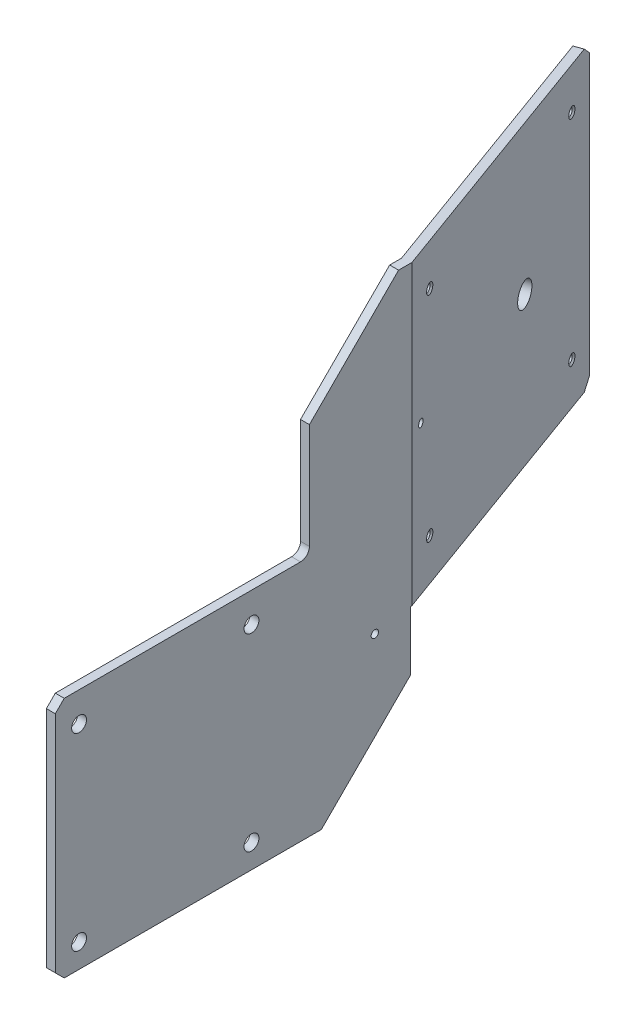
from build123d import *

# Parameters (mm, degrees)
BOSS_EXTRUDE1_DEPTH   = 100
SKETCH3_R             = 1
CUT_EXTRUDE2_DEPTH    = 10
LPATTERN1_COUNT       = 2
LPATTERN1_PITCH       = 80
M3_TAPPED_HOLE1_D     = 2.5
M3_TAPPED_HOLE1_DEPTH = 7.5
M3_TAPPED_HOLE1_TIP   = 0.751075774
CHAMFER2_SIZE         = 0.5
SKETCH6_W             = 85.5
SKETCH6_H             = 68.5
CUT_EXTRUDE4_DEPTH    = 10
CHAMFER3_SIZE         = 30
FILLET1_R             = 3
SKETCH7_R             = 4
CUT_EXTRUDE5_DEPTH    = 10
SKETCH9_W             = 119.5
SKETCH9_H             = 50
BOSS_EXTRUDE2_DEPTH   = 3
SKETCH5_R             = 2.5
CUT_EXTRUDE3_DEPTH    = 10
CHAMFER4_SIZE         = 3
CHAMFER5_SIZE         = 30
M3_TAPPED_HOLE2_D     = 2.5
M3_TAPPED_HOLE2_DEPTH = 7.5
M3_TAPPED_HOLE2_TIP   = 0.751075774
M3_TAPPED_HOLE3_D     = 2.5
M3_TAPPED_HOLE3_DEPTH = 7.5
M3_TAPPED_HOLE3_TIP   = 0.751075774


with BuildPart() as part:
    # Sketch1 → Boss-Extrude1 (new body)
    with BuildSketch(Plane(origin=(0, 0, 0), x_dir=(1, 0, 0), z_dir=(0, 1, 0))):
        Polygon((0, 120), (-34.202014333, 213.969262079), (-37.021092195, 212.943201649), (-3, 119.471019058), (-3, 0), (0, 0), align=None)
    extrude(amount=BOSS_EXTRUDE1_DEPTH)

    # Sketch3 → Cut-Extrude2 (cut)
    with BuildSketch(Plane(origin=(35.748178719, 0, -13.011272983), x_dir=(0.3420201433256699, 0, 0.939692620785908), z_dir=(-0.9396926207859081, 0, 0.3420201433256699))):
        with Locations((-202.763114494, 86)):
            Circle(SKETCH3_R)
        with Locations((-202.763114494, 14)):
            Circle(SKETCH3_R)
    cut_extrude2 = extrude(amount=-CUT_EXTRUDE2_DEPTH, mode=Mode.SUBTRACT)

    # LPattern1: Cut-Extrude2 ×2
    with Locations(*[Vector(0.3420201433256699, 0, 0.939692620785908) * (i * LPATTERN1_PITCH) for i in range(1, LPATTERN1_COUNT)]):
        add(cut_extrude2, mode=Mode.SUBTRACT)

    # M3 Tapped Hole1
    with Locations(Plane(origin=(-30.781812899, 86, -204.572335871), x_dir=(0.342020143326, 0, 0.939692620786), z_dir=(0.939692620786, 0, -0.342020143326))):
        with Locations((0, 0), (0, 72), (80, 72), (80, 0)):
            Hole(M3_TAPPED_HOLE1_D / 2, depth=M3_TAPPED_HOLE1_DEPTH)
            with Locations((0, 0, -(M3_TAPPED_HOLE1_DEPTH + M3_TAPPED_HOLE1_TIP / 2))):  # 118° drill point
                Cone(0, M3_TAPPED_HOLE1_D / 2, M3_TAPPED_HOLE1_TIP, mode=Mode.SUBTRACT)

    # Chamfer2
    chamfer2_edges = [part.edges().sort_by_distance(p)[0] for p in [
        (-2.992676254, 86, -128.222310432),
        (-2.992676254, 14, -128.222310432),
        (-30.35428772, 14, -203.397720095),
        (-30.35428772, 86, -203.397720095),
    ]]
    chamfer(chamfer2_edges, length=CHAMFER2_SIZE)

    # Sketch6 → Cut-Extrude4 (cut)
    with BuildSketch(Plane.ZY.offset(3)):
        with Locations((-42.75, 65.75)):
            Rectangle(SKETCH6_W, SKETCH6_H)
    extrude(amount=-CUT_EXTRUDE4_DEPTH, mode=Mode.SUBTRACT)

    # Chamfer3
    chamfer3_edges = [part.edges().sort_by_distance(p)[0] for p in [
        (-1.5, 100, -85.5),
    ]]
    chamfer(chamfer3_edges, length=CHAMFER3_SIZE)

    # Fillet1
    fillet1_edges = [part.edges().sort_by_distance(p)[0] for p in [
        (-1.5, 31.5, -85.5),
    ]]
    fillet(fillet1_edges, radius=FILLET1_R)

    # Sketch7 → Cut-Extrude5 (cut)
    with BuildSketch(Plane(origin=(35.748178719, 0, -13.011272983), x_dir=(0.3420201433256699, 0, 0.939692620785908), z_dir=(-0.9396926207859081, 0, 0.3420201433256699))):
        with Locations((-176.263114494, 50)):
            Circle(SKETCH7_R)
    extrude(amount=-CUT_EXTRUDE5_DEPTH, mode=Mode.SUBTRACT)

    # Sketch9 → Boss-Extrude2 (add)
    with BuildSketch(Plane.ZY.offset(3)):
        with Locations((-59.75, -25)):
            Rectangle(SKETCH9_W, SKETCH9_H)
    extrude(amount=-BOSS_EXTRUDE2_DEPTH)

    # Sketch5 → Cut-Extrude3 (cut)
    with BuildSketch(Plane.ZY.offset(3)):
        with Locations((-8, 21.5)):
            Circle(SKETCH5_R)
        with Locations((-8, -42)):
            Circle(SKETCH5_R)
        with Locations((-66, 21.5)):
            Circle(SKETCH5_R)
        with Locations((-66, -42)):
            Circle(SKETCH5_R)
    extrude(amount=-CUT_EXTRUDE3_DEPTH, mode=Mode.SUBTRACT)

    # Chamfer4
    chamfer4_edges = [part.edges().sort_by_distance(p)[0] for p in [
        (-1.5, 31.5, 0),
        (-35.611553264, 100, -213.456231864),
        (-35.611553264, 0, -213.456231864),
        (-1.5, -50, 0),
    ]]
    chamfer(chamfer4_edges, length=CHAMFER4_SIZE)

    # Chamfer5
    chamfer5_edges = [part.edges().sort_by_distance(p)[0] for p in [
        (-1.5, -50, -119.5),
    ]]
    chamfer(chamfer5_edges, length=CHAMFER5_SIZE)

    # M3 Tapped Hole2
    with Locations(Plane(origin=(35.748178719, 0, -13.011272983), x_dir=(0.3420201433256699, 0, 0.939692620785908), z_dir=(-0.9396926207859081, 0, 0.3420201433256699))):
        with Locations((-117.763114494, 50)):
            Hole(M3_TAPPED_HOLE2_D / 2, depth=M3_TAPPED_HOLE2_DEPTH)
            with Locations((0, 0, -(M3_TAPPED_HOLE2_DEPTH + M3_TAPPED_HOLE2_TIP / 2))):  # 118° drill point
                Cone(0, M3_TAPPED_HOLE2_D / 2, M3_TAPPED_HOLE2_TIP, mode=Mode.SUBTRACT)

    # M3 Tapped Hole3
    with Locations(Plane.ZY.offset(3)):
        with Locations((-107.5, -2)):
            Hole(M3_TAPPED_HOLE3_D / 2, depth=M3_TAPPED_HOLE3_DEPTH)
            with Locations((0, 0, -(M3_TAPPED_HOLE3_DEPTH + M3_TAPPED_HOLE3_TIP / 2))):  # 118° drill point
                Cone(0, M3_TAPPED_HOLE3_D / 2, M3_TAPPED_HOLE3_TIP, mode=Mode.SUBTRACT)


solid = part.part
